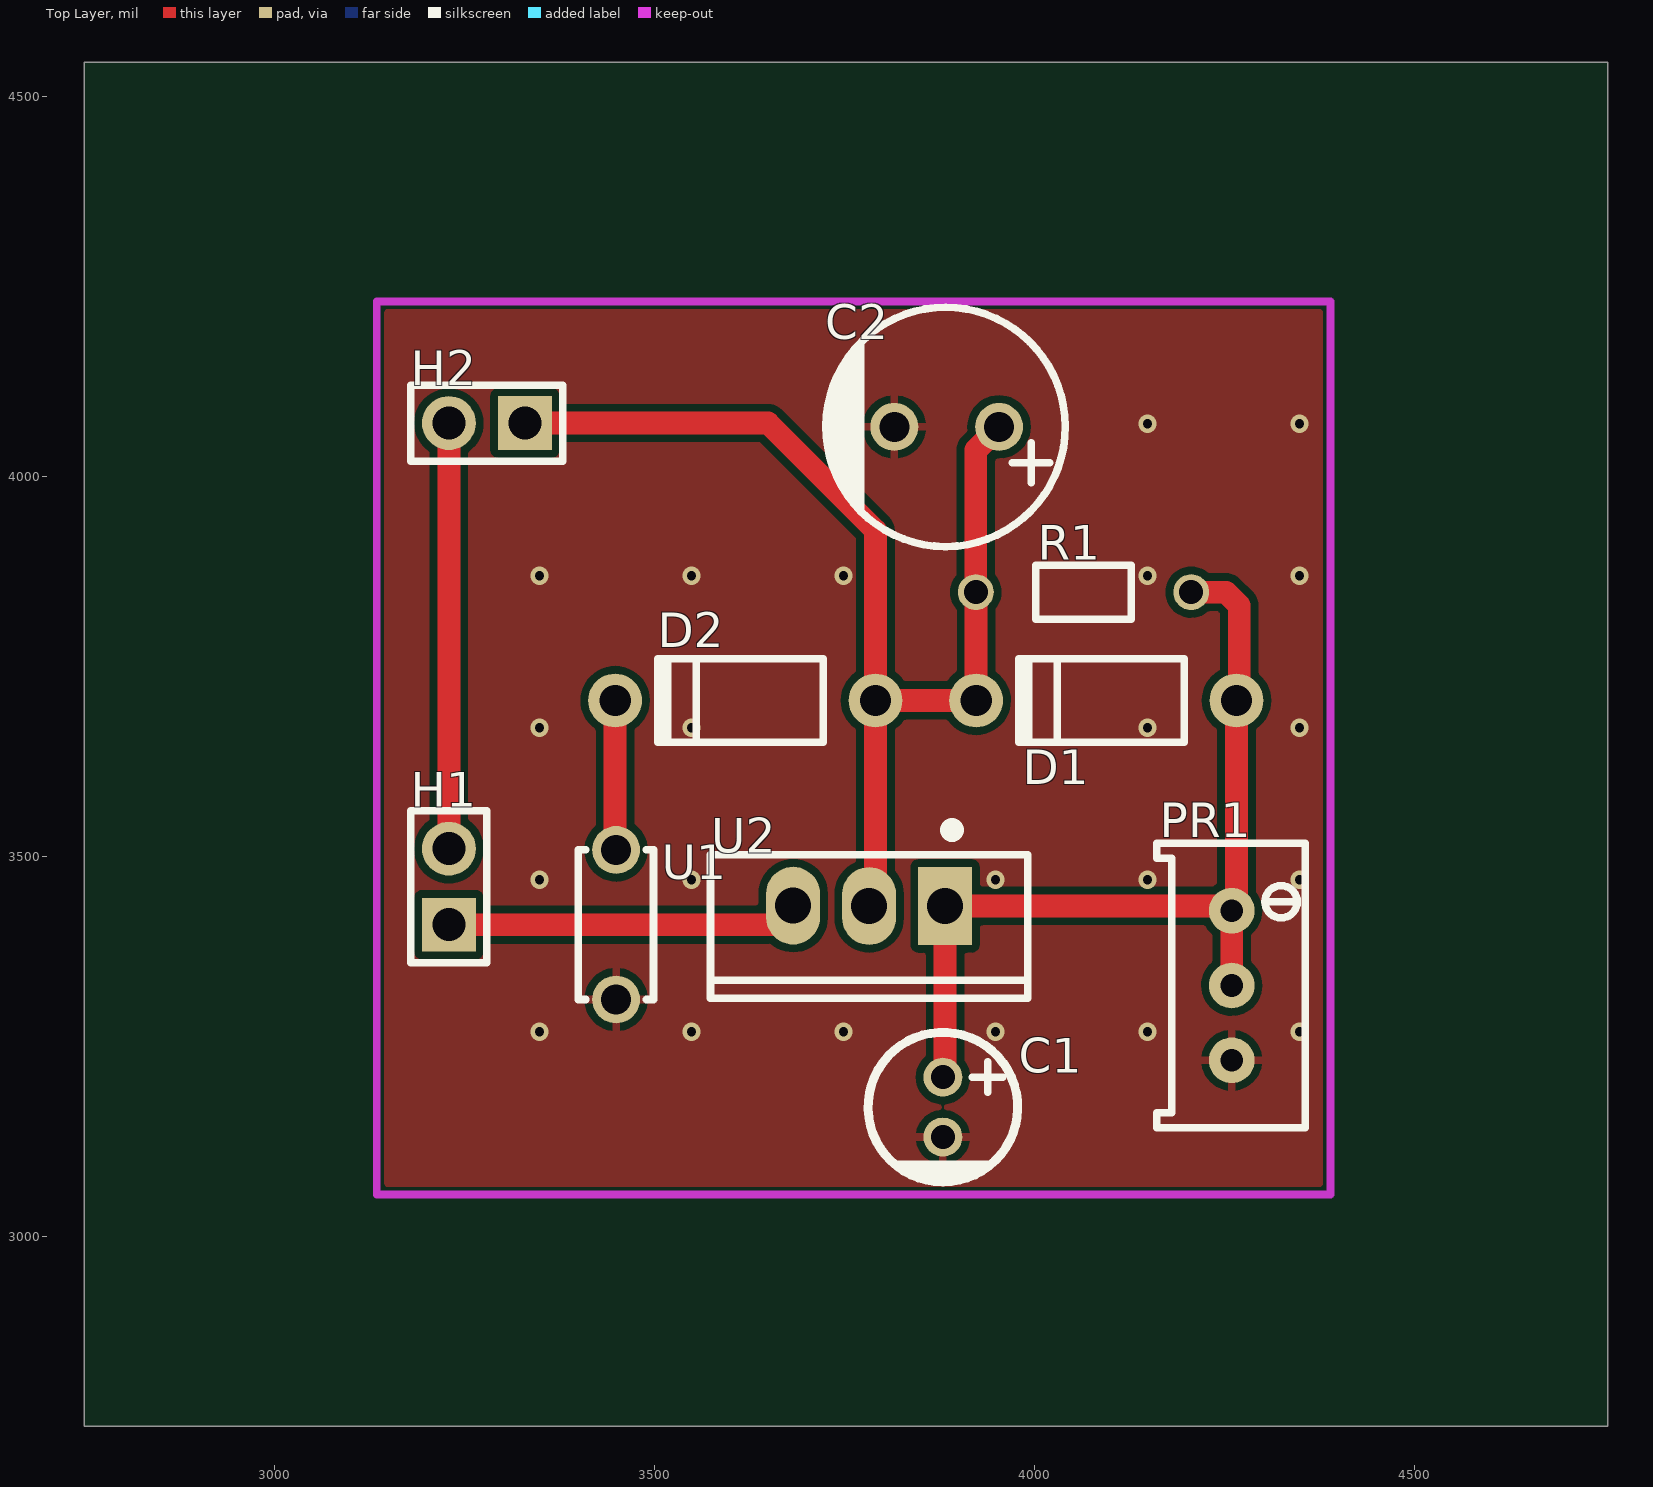
[diagram p0: Top Layer view]
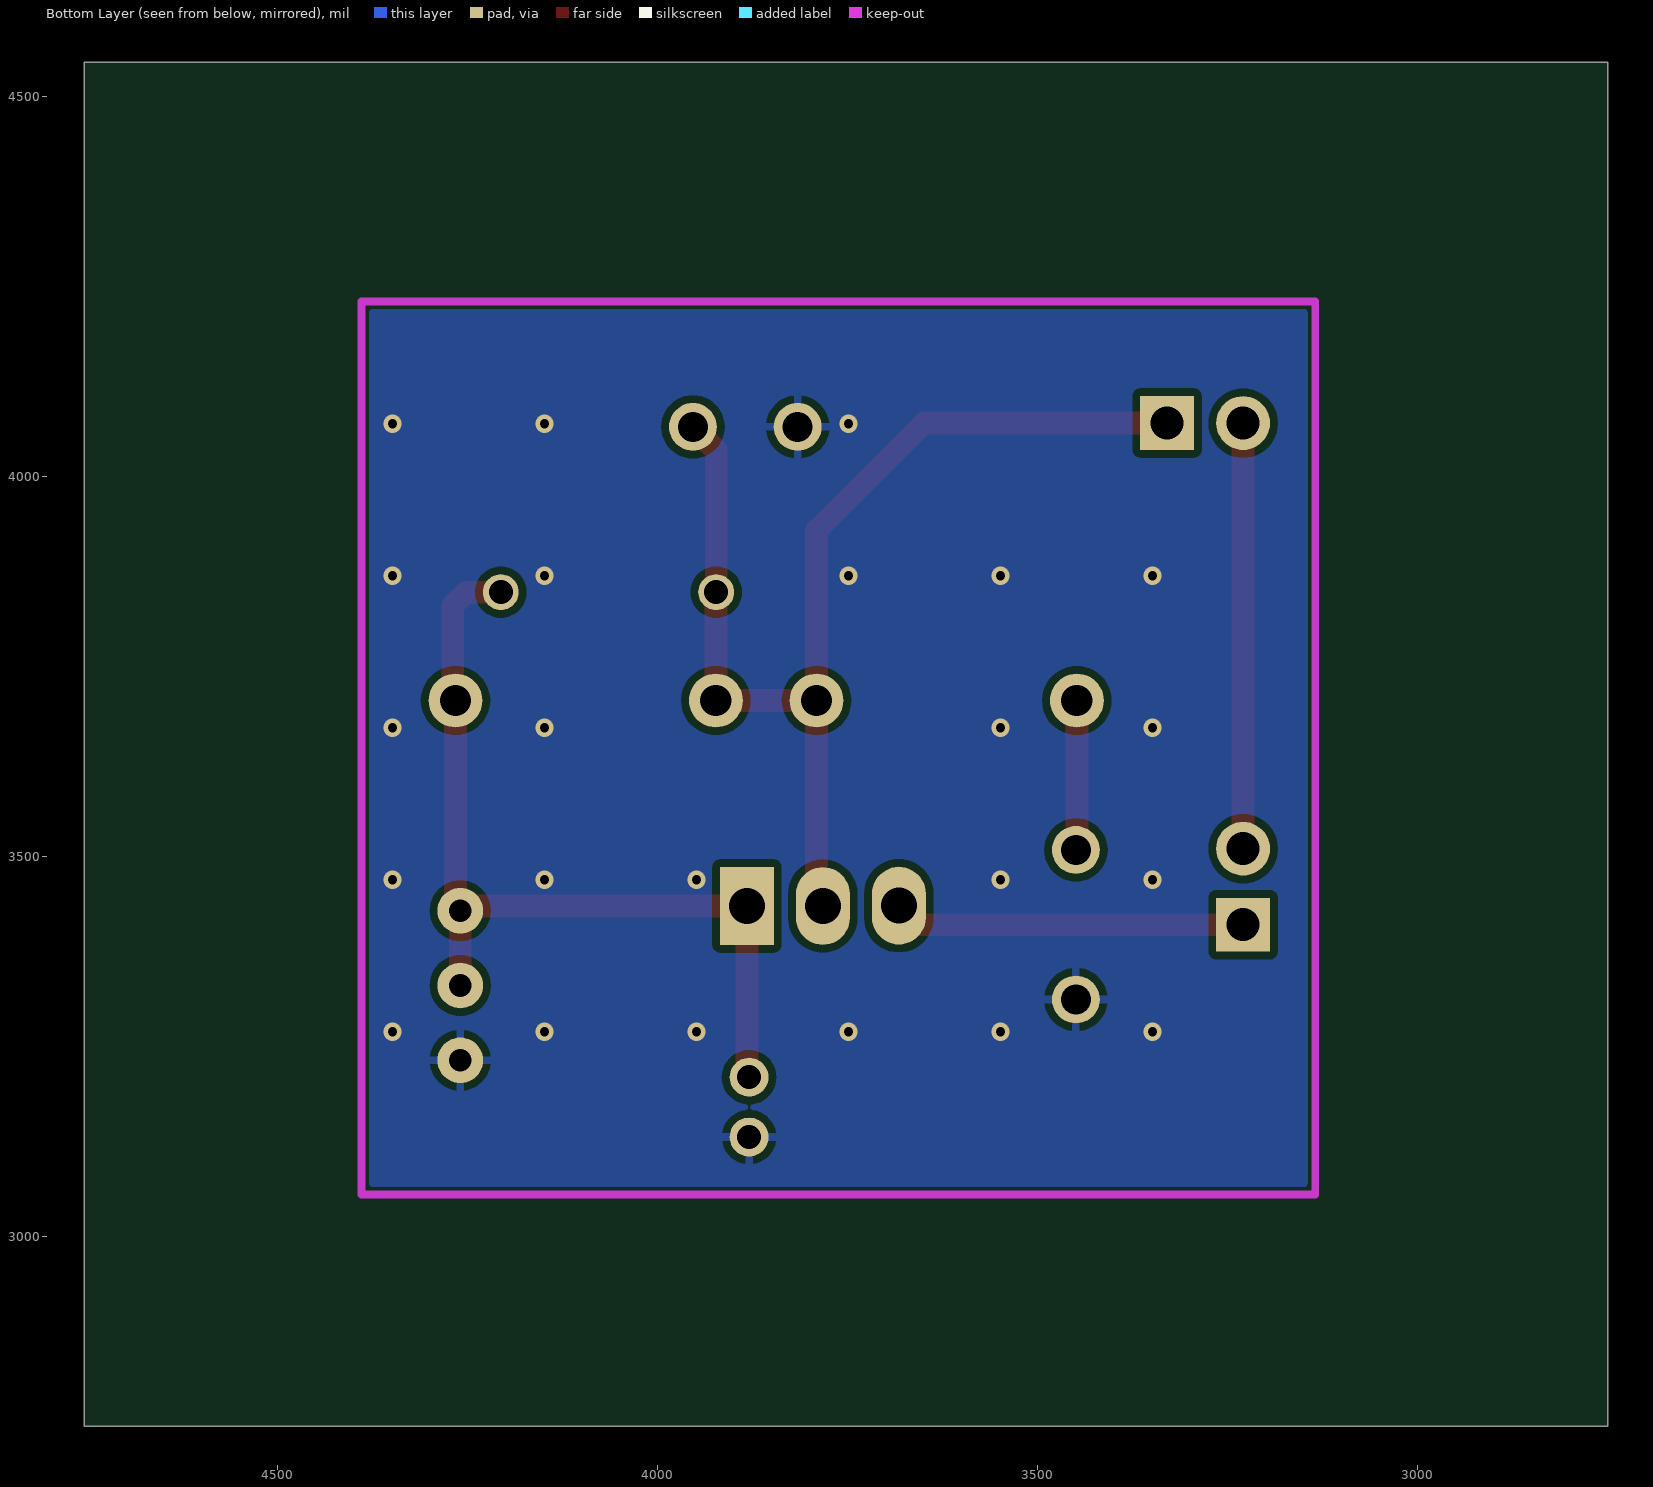
[diagram p1: Bottom Layer view, seen from below]
# Altium PCB MISC49891.pcbdoc
Units mil, origin at the board's own origin, x right, y up, seen from the top; angles counter-clockwise.
Board outline 2005 x 1795 mil, 2 copper layers (Top Layer, Bottom Layer), stack 62.206 mil thick; 10 components, 6 nets, 22 pads, 23 vias.

## Layer stack, top to bottom
Top Solder Mask Layer: solder mask 0.394, Dk 3.3
Top Layer: signal copper 1.379
Dielectric1: surface 59.449, FR4, Dk 4.5
Bottom Layer: signal copper 1.378
Bottom Solder Mask Layer: solder mask 0.394, Dk 3.3

## Board outline
4755,2750 2750,2750 2750,4545 4755,4545

## Design rules (kind name [scope] priority, off if disabled: settings)
BoardOutlineClearance copperThickness2oz_1 [All] p2 off: genericclearance=7.99 ignorepadtopadclearanceinfootprint=FALSE except(0: Arc-SplitContinuation Track-SplitContinuation SMDPad-SplitContinuation THPad-SplitContinuation Via-SplitContinuation Fill-SplitContinuation Region-SplitContinuation Poly-SplitContinuation Text-SplitContinuation Hole-SplitContinuation; 5.98: Arc-CutoutEdge SMDPad-CutoutEdge THPad-CutoutEdge Via-CutoutEdge Fill-CutoutEdge Region-CutoutEdge Text-CutoutEdge; 6.93: Hole-OutlineEdge Hole-CutoutEdge; 10: Poly-OutlineEdge Poly-CutoutEdge; 11.81: Arc-OutlineEdge Track-OutlineEdge SMDPad-OutlineEdge THPad-OutlineEdge Via-OutlineEdge Fill-OutlineEdge Region-OutlineEdge Text-OutlineEdge Track-CutoutEdge)
BoardOutlineClearance copperThickness1oz_1 [All] p4: genericclearance=4.02 ignorepadtopadclearanceinfootprint=FALSE except(0: Arc-SplitContinuation Track-SplitContinuation SMDPad-SplitContinuation THPad-SplitContinuation Via-SplitContinuation Fill-SplitContinuation Region-SplitContinuation Poly-SplitContinuation Text-SplitContinuation Hole-SplitContinuation; 6: SMDPad-CutoutEdge THPad-CutoutEdge Via-CutoutEdge Fill-CutoutEdge Region-CutoutEdge Text-CutoutEdge; 6.93: Hole-OutlineEdge Hole-CutoutEdge; 10: Poly-OutlineEdge Poly-CutoutEdge; 11.8: Arc-OutlineEdge Track-OutlineEdge SMDPad-OutlineEdge THPad-OutlineEdge Via-OutlineEdge Fill-OutlineEdge Region-OutlineEdge Text-OutlineEdge; 11.81: Arc-CutoutEdge Track-CutoutEdge)
Clearance copperThickness2oz [All] p1 off: gap=7.99 ignorepadtopadclearanceinfootprint=FALSE except(5.98: SMDPad-Track SMDPad-SMDPad THPad-Track SMDPad-THPad THPad-THPad Track-Via SMDPad-Via THPad-Via Via-Via Fill-Track Region-Track Fill-SMDPad Region-SMDPad Fill-THPad Region-THPad Fill-Via Region-Via Fill-Fill Fill-Region Region-Region Arc-Track Arc-SMDPad Arc-THPad Arc-Via Fill-Arc Region-Arc Arc-Arc Text-Track SMDPad-Text Text-THPad Text-Via Fill-Text Region-Text Arc-Text Text-Text; 6.93: Hole-Track Hole-SMDPad Hole-THPad Hole-Via Fill-Hole Region-Hole Hole-Arc Hole-Text; 10: Poly-Track Poly-SMDPad Poly-THPad Poly-Via Poly-Fill Poly-Region Poly-Poly Poly-Arc Poly-Text Poly-Hole)
Clearance copperThickness1oz [All] p3: gap=4.02 ignorepadtopadclearanceinfootprint=FALSE except(5.98: SMDPad-Track SMDPad-SMDPad THPad-Track SMDPad-THPad THPad-THPad Track-Via SMDPad-Via THPad-Via Via-Via Fill-Track Region-Track Fill-SMDPad Region-SMDPad Fill-THPad Region-THPad Fill-Via Region-Via Fill-Fill Fill-Region Region-Region; 6: Arc-Track Arc-SMDPad Arc-THPad Arc-Via Fill-Arc Region-Arc Arc-Arc Text-Track SMDPad-Text Text-THPad Text-Via Fill-Text Region-Text Arc-Text Text-Text; 6.93: Hole-Track Hole-SMDPad Hole-THPad Hole-Via Fill-Hole Region-Hole Hole-Arc Hole-Text; 10: Poly-Track Poly-SMDPad Poly-THPad Poly-Via Poly-Fill Poly-Region Poly-Poly Poly-Arc Poly-Text Poly-Hole)
DiffPairsRouting differentialPair [All] p1: maxlimit=6 minlimit=6 mostfreqgap=6 toplayer_minwidth=5 toplayer_prefwidth=10 toplayer_maxwidth=100 toplayer_mingap=6 toplayer_prefgap=6 toplayer_maxgap=6 bottomlayer_minwidth=5 bottomlayer_prefwidth=10 bottomlayer_maxwidth=100 bottomlayer_mingap=6 bottomlayer_prefgap=6 bottomlayer_maxgap=6 maxuncoupledlength=10
HoleToHoleClearance otherClearance [All] p1: gap=11.81 allowstackedmicrovias=TRUE
Length netLength [All] p1: minlimit=0 maxlimit=0
MatchedLengths netLengthTolerance [All] p1: tolerance=1000
PasteMaskExpansion pasteMaskExpansion [All] p1: expansion=0
PlaneConnect innerPlane [All] p1: planeconnectstyle=Relief reliefexpansion=20 reliefentries=4 reliefconductorwidth=10 reliefairgap=10
PolygonConnect copperRegion [(InNet('GND'))] p1: connectstyle=Relief reliefconductorwidth=10 reliefentries=4 polygonreliefangle="90 Angle" airgapwidth=10 via.connectstyle=Relief via.reliefconductorwidth=10 via.reliefentries=4 via.polygonreliefangle="90 Angle" via.airgapwidth=10
RoutingVias viaSize [All] p1: holewidth=12.01 width=24.02 viastyle="Through Hole" minholewidth=11.81 minwidth=19.68 maxholewidth=248.03 maxwidth=393.7
SolderMaskExpansion solderMaskExpansion [IsVia] p1: expansion=-1000 istentingtop=TRUE
SolderMaskExpansion solderMaskExpansion [All] p2: expansion=2 istentingtop=FALSE
Width copperThickness2oz_2 [All] p1 off: maxlimit=100 minlimit=8 preferedwidth=10
Width copperThickness1oz_2 [All] p2: maxlimit=100 minlimit=5 preferedwidth=10

## Components (designator, comment, footprint, x,y, rotation, side; value= is the part's Value field where it differs from the comment)
C1 "10uF" CAP-TH_BD5.0-P2.00-D0.8-FD-10UF50VC110GL 3880,3170 r270 top
C2 "100uF" CAP-TH_BD8.0-P3.50-D0.6-FD_1 3885,4065 r180 top
D1 "1N4001" DO-41_BD2.4-L4.7-P8.70-D0.8-RD 4095,3705 r0 top
D2 "1N4001" DO-41_BD2.4-L4.7-P8.70-D0.8-RD 3620,3705 r0 top
H1 "" HDR-TH_2P-P2.54-V-M-1 3230,3460 r90 top
H2 "" HDR-TH_2P-P2.54-V-M-1 3280,4070 r180 top
PR1 "10kΩ" R_3296 4265,3330 r270 top
R1 "200Ω" Res_1/8W 4065,3850 r180 top
U1 "2.2nF" CAP-TH_L5.0-W2.5-P5.00-D1.0 3450,3410 r270 top
U2 "LM317AHVT" TO-220-3_L10.0-W4.5-P2.54-L 3782.92,3434.88 r180 top

## Footprints (in the part's own frame and the unit in brackets; to place one, negate y for a bottom-side part, rotate by r counter-clockwise, add the part's x,y. Pads: shape width x height; smd on the part's side, far side on the other; paste and mask are expansions set on the pad)
CAP-TH_BD5.0-P2.00-D0.8-FD-10UF50VC110GL [mm]
  round 1.3 hole 0.8: 1(-1,0) 2(1,0)
  silkscreen extent -2.5,-2.5 2.5,2.5
CAP-TH_BD8.0-P3.50-D0.6-FD_1 [mm]
  round 1.6 hole 1: 1(-1.75,0) 2(1.75,0)
  silkscreen extent -3.96,-4 4.04,4
CAP-TH_L5.0-W2.5-P5.00-D1.0 [mm]
  round 1.6 hole 1: 1(-2.5,0) 2(2.5,0)
  silkscreen extent -2.5,-1.27 2.5,1.25
DO-41_BD2.4-L4.7-P8.70-D0.8-RD [mm]
  round 1.8 hole 1.05: 1(-4.35,0) 2(4.35,0)
  silkscreen extent -2.92,-1.4 2.6,1.4
HDR-TH_2P-P2.54-V-M-1 [mm]
  rect 1.8x1.8 hole 1.1: 1(-1.27,0)
  round 1.8 hole 1.1: 2(1.27,0)
  silkscreen extent -2.54,-1.27 2.54,1.27
R_3296 [mil]
  round 60 hole 30 paste+0 mask+2: 1(-98.4,-5) 2(0,-5) 3(98.4,-5)
  silkscreen extent -187,-103 187,92
Res_1/8W [mil]
  round 47.2 hole 31.5 paste+0 mask+2: 1(-141.7,2.48) 2(141.7,2.48)
  silkscreen extent -63,-33 63,38
TO-220-3_L10.0-W4.5-P2.54-L [mm]
  rect 1.8x2.6 hole 1.2: 1(-2.54,0.005)
  oval 1.8x2.6 hole 1.2: 2(0,0.005)
  oval 1.8x2.6 hole 1.2 copper offset 0,0: 3(2.54,-0.005)
  silkscreen extent -5.3,-2.73 5.3,3.09

## Via types
v1: diameter 24.02, hole 12, Top Layer to Bottom Layer, 23 vias

## Nets (pads, with @x,y where several pads share a name; then routed paths per layer and width w, separated by ;. In a path a pad name is that pad's centre, name@x,y a point inside that pad or via, vN(x,y) a via of type N, cw(c..) or ccw(c..) an arc to the next point about the centre after c; other vN are vias at no path point)
$1N1: C1.1 D1.2 PR1.1 PR1.2 R1.1 U2.1 | length 1180.9
  Top Layer w30: C1.1 3882.92,3212.29 U2.1 4253.71,3434.69 PR1.1 ; R1.1 4252.48,3847.52 4270,3830 4270,3708.74 D1.2 4266.26,3434.66 PR1.1 ; PR1.2 PR1.1
$1N2: C2.1 D1.1 D2.2 H2.1 R1.2 U2.2 | length 1522.6
  Top Layer w30: H2.1 3650,4070 3791.26,3928.74 D2.2 ; U2.2 3791.26,3443.02 D2.2 ; C2.1 3923.3,4034.4 R1.2 3923.74,3847.08 D1.1 D2.2
$1N5: D2.1 U1.1 | length 197.1
  Top Layer w30: D2.1 3448.74,3509.68 U1.1
$1N6: H1.1 U2.3 | length 463.3
  Top Layer w30: H1.1 3657.84,3410 U2.3
$1N7: H1.2 H2.2 | length 560
  Top Layer w30: H1.2 H2.2
GND: C1.2 C2.2 PR1.3 U1.2
  other v1: 3349.1,3269.1 3549.1,3269.1 3749.1,3269.1 3949.1,3269.1 4149.1,3269.1 4349.1,3269.1 3349.1,3469.1 3549.1,3469.1 3949.1,3469.1 4149.1,3469.1 4349.1,3469.1 3349.1,3669.1 3549.1,3669.1 4149.1,3669.1 4349.1,3669.1 3349.1,3869.1 3549.1,3869.1 3749.1,3869.1 4149.1,3869.1 4349.1,3869.1 3749.1,4069.1 4149.1,4069.1 4349.1,4069.1

## Polygon pours and split planes (outlines as drawn)
GND on Top Layer (solid, remove dead copper, pour order 0): 3000,4295 3000,3000 4505,3000 4505,4295
GND on Bottom Layer (solid, remove dead copper, pour order 2): 3080,4280 3080,3015 4470,3015 4470,4280

## Keep-outs
Board Outline Layer:
  lines w10: 3135,3055 3135,4230 4390,4230 4390,3055 3135,3055